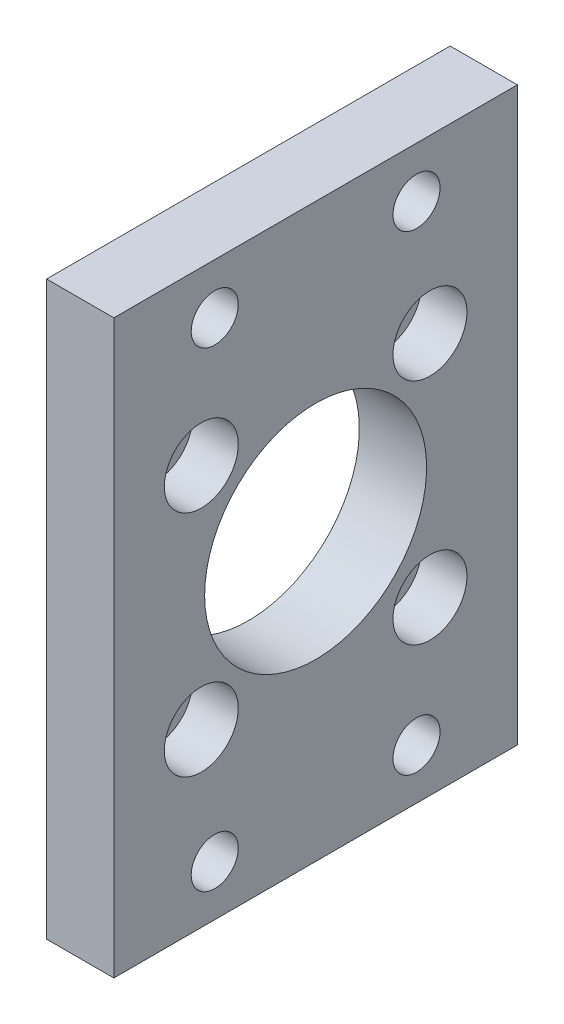
from build123d import *

# Parameters (mm, degrees)
SKETCH_1_W                = 60
SKETCH_1_H                = 85
EXTRUDE_1_DEPTH           = 10
HOLE_WIZARD_1_D           = 6.6
HOLE_WIZARD_1_CBORE_D     = 11
HOLE_WIZARD_1_CBORE_DEPTH = 6.8
HOLE_WIZARD_7_0_7_1_D     = 7
SKETCH_6_R                = 16.5
CUT_EXTRUDE_1_DEPTH       = 53.974050251


with BuildPart() as part:
    # 草图1 → 凸台-拉伸1 (new body)
    with BuildSketch(Plane(origin=(0, 0, 0), x_dir=(0, 0, -1), z_dir=(1, 0, 0))):
        Rectangle(SKETCH_1_W, SKETCH_1_H)
    extrude(amount=EXTRUDE_1_DEPTH)

    # 打孔尺寸(%根据)内六角圆柱头螺钉的类型1 (through all)
    with Locations(Plane(origin=(10, 0, 0), x_dir=(0, 0, -1), z_dir=(1, 0, 0))):
        with Locations((-17, 17), (17, 17), (-17, -17), (17, -17)):
            CounterBoreHole(HOLE_WIZARD_1_D / 2, HOLE_WIZARD_1_CBORE_D / 2, HOLE_WIZARD_1_CBORE_DEPTH)

    # Ø7.0 (7) 直径孔1 (through all)
    with Locations(Plane.ZY):
        with Locations((-15, 35), (15, 35), (-15, -35), (15, -35)):
            Hole(HOLE_WIZARD_7_0_7_1_D / 2)

    # 草图6 → 切除-拉伸1 (cut, through all)
    with BuildSketch(Plane.ZY):
        Circle(SKETCH_6_R)
    extrude(amount=-CUT_EXTRUDE_1_DEPTH, mode=Mode.SUBTRACT)


solid = part.part
